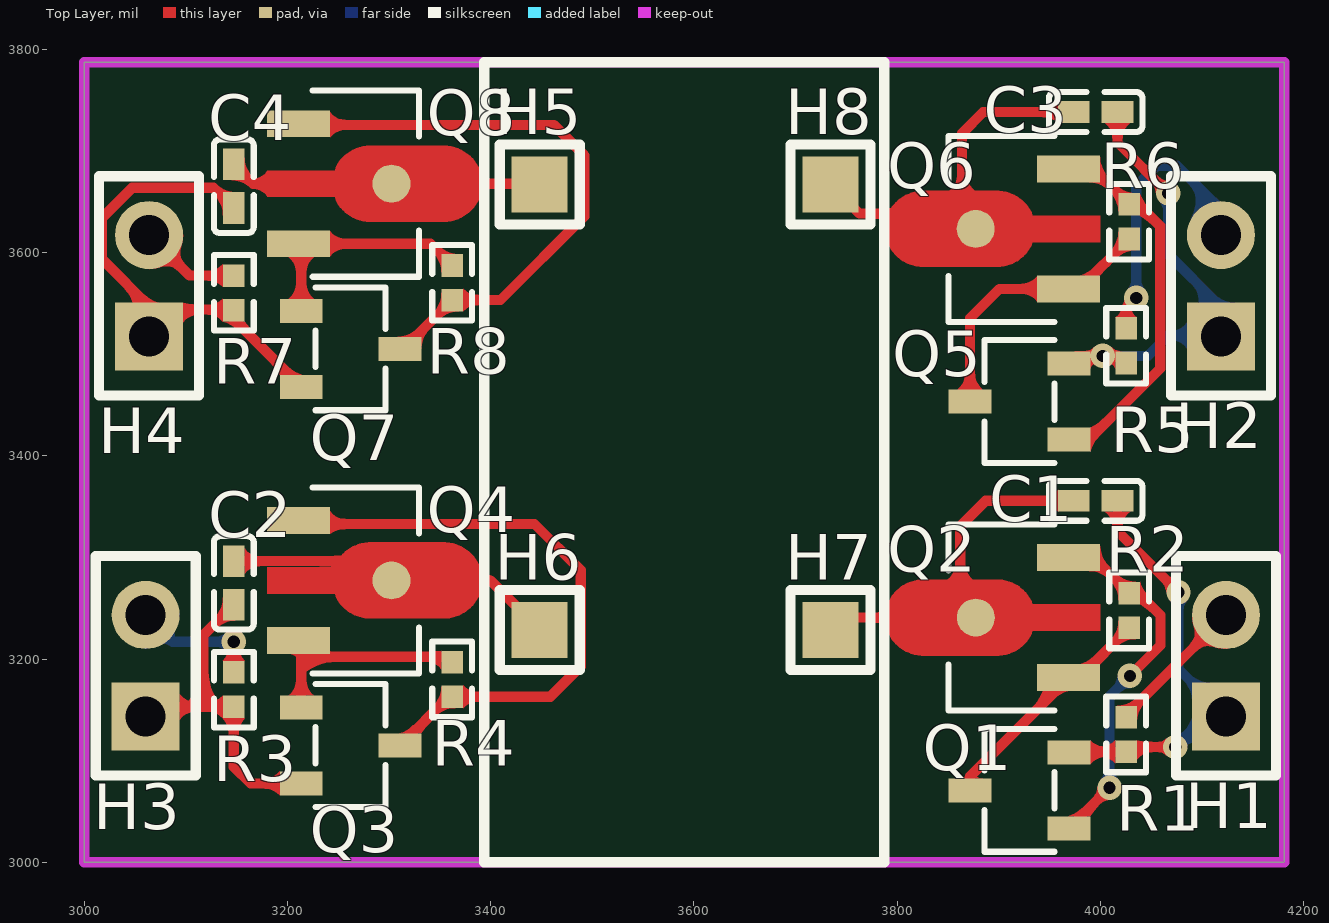
[diagram p0: Top Layer view]
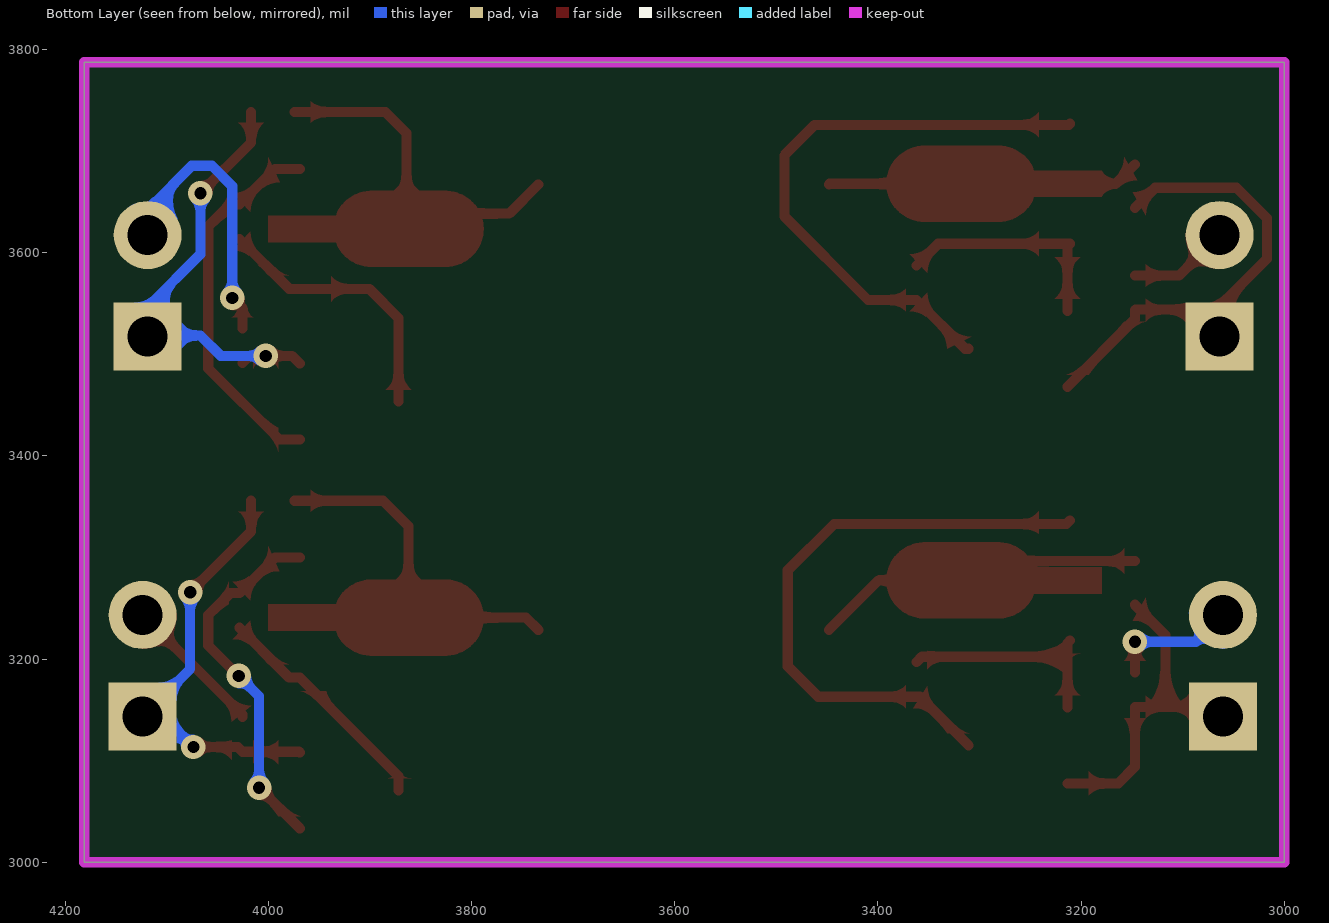
[diagram p1: Bottom Layer view, seen from below]
# Altium PCB MISC51349.pcbdoc
Units mil, origin at the board's own origin, x right, y up, seen from the top; angles counter-clockwise.
Board outline 1181.1 x 787.4 mil, 2 copper layers (Top Layer, Bottom Layer), stack 62.206 mil thick; 28 components, 20 nets, 60 pads, 8 vias.

## Layer stack, top to bottom
Top Solder Mask Layer: solder mask 0.394, Dk 3.3
Top Layer: signal copper 1.379
Dielectric1: surface 59.449, FR4, Dk 4.5
Bottom Layer: signal copper 1.378
Bottom Solder Mask Layer: solder mask 0.394, Dk 3.3

## Board outline
4181.1,3787.4 3000,3787.4 3000,3000 4181.1,3000

## Design rules (kind name [scope] priority, off if disabled: settings)
BoardOutlineClearance copperThickness2oz_1 [All] p2 off: genericclearance=7.99 ignorepadtopadclearanceinfootprint=FALSE except(0: Arc-SplitContinuation Track-SplitContinuation SMDPad-SplitContinuation THPad-SplitContinuation Via-SplitContinuation Fill-SplitContinuation Region-SplitContinuation Poly-SplitContinuation Text-SplitContinuation Hole-SplitContinuation; 5.98: Arc-CutoutEdge Track-CutoutEdge SMDPad-CutoutEdge THPad-CutoutEdge Via-CutoutEdge Text-CutoutEdge; 6.9: Hole-OutlineEdge Hole-CutoutEdge; 10: Poly-OutlineEdge Poly-CutoutEdge; 11.81: Arc-OutlineEdge Track-OutlineEdge SMDPad-OutlineEdge THPad-OutlineEdge Via-OutlineEdge Fill-OutlineEdge Region-OutlineEdge Text-OutlineEdge Fill-CutoutEdge Region-CutoutEdge)
BoardOutlineClearance Plane_innerPlane_1 [All] p4 off: genericclearance=4.02 ignorepadtopadclearanceinfootprint=FALSE except(0: Arc-SplitContinuation Track-SplitContinuation SMDPad-SplitContinuation THPad-SplitContinuation Via-SplitContinuation Fill-SplitContinuation Region-SplitContinuation Poly-SplitContinuation Text-SplitContinuation Hole-SplitContinuation; 5.98: Arc-CutoutEdge Track-CutoutEdge SMDPad-CutoutEdge THPad-CutoutEdge Via-CutoutEdge Text-CutoutEdge; 6.9: Hole-OutlineEdge Hole-CutoutEdge; 10: Poly-OutlineEdge Poly-CutoutEdge; 11.81: Arc-OutlineEdge Track-OutlineEdge SMDPad-OutlineEdge THPad-OutlineEdge Via-OutlineEdge Fill-OutlineEdge Region-OutlineEdge Text-OutlineEdge Fill-CutoutEdge Region-CutoutEdge)
BoardOutlineClearance Copper_copperRegion_1 [All] p6 off: genericclearance=4.02 ignorepadtopadclearanceinfootprint=FALSE except(0: Arc-SplitContinuation Track-SplitContinuation SMDPad-SplitContinuation THPad-SplitContinuation Via-SplitContinuation Fill-SplitContinuation Region-SplitContinuation Poly-SplitContinuation Text-SplitContinuation Hole-SplitContinuation; 5.98: Arc-CutoutEdge Track-CutoutEdge SMDPad-CutoutEdge THPad-CutoutEdge Via-CutoutEdge Text-CutoutEdge; 6.9: Hole-OutlineEdge Hole-CutoutEdge; 10: Poly-OutlineEdge Poly-CutoutEdge; 11.81: Arc-OutlineEdge Track-OutlineEdge SMDPad-OutlineEdge THPad-OutlineEdge Via-OutlineEdge Fill-OutlineEdge Region-OutlineEdge Text-OutlineEdge Fill-CutoutEdge Region-CutoutEdge)
BoardOutlineClearance copperThickness1oz_1 [All] p8: genericclearance=4.02 ignorepadtopadclearanceinfootprint=FALSE except(0: Arc-SplitContinuation Track-SplitContinuation SMDPad-SplitContinuation THPad-SplitContinuation Via-SplitContinuation Fill-SplitContinuation Region-SplitContinuation Poly-SplitContinuation Text-SplitContinuation Hole-SplitContinuation; 5.98: Arc-CutoutEdge Track-CutoutEdge SMDPad-CutoutEdge THPad-CutoutEdge Via-CutoutEdge Text-CutoutEdge; 6.9: Hole-OutlineEdge Hole-CutoutEdge; 10: Poly-OutlineEdge Poly-CutoutEdge; 11.81: Arc-OutlineEdge Track-OutlineEdge SMDPad-OutlineEdge THPad-OutlineEdge Via-OutlineEdge Fill-OutlineEdge Region-OutlineEdge Text-OutlineEdge Fill-CutoutEdge Region-CutoutEdge)
Clearance copperThickness2oz [All] p1 off: gap=7.99 ignorepadtopadclearanceinfootprint=FALSE except(5.98: SMDPad-Track SMDPad-SMDPad THPad-Track SMDPad-THPad THPad-THPad Track-Via SMDPad-Via THPad-Via Via-Via Fill-SMDPad Region-SMDPad Fill-THPad Region-THPad Fill-Via Region-Via Fill-Fill Fill-Region Region-Region Arc-Track Arc-SMDPad Arc-THPad Arc-Via Fill-Arc Region-Arc Arc-Arc Text-Track SMDPad-Text Text-THPad Text-Via Fill-Text Region-Text Arc-Text Text-Text; 6.9: Hole-Track Hole-SMDPad Hole-THPad Hole-Via Fill-Hole Region-Hole Hole-Arc Hole-Text; 10: Poly-Track Poly-SMDPad Poly-THPad Poly-Via Poly-Fill Poly-Region Poly-Poly Poly-Arc Poly-Text Poly-Hole; 11.81: Fill-Track Region-Track)
Clearance Plane_innerPlane [All] p3 off: gap=4.02 ignorepadtopadclearanceinfootprint=FALSE except(5.98: SMDPad-Track SMDPad-SMDPad THPad-Track SMDPad-THPad THPad-THPad Track-Via SMDPad-Via THPad-Via Via-Via Fill-SMDPad Region-SMDPad Fill-THPad Region-THPad Fill-Via Region-Via Fill-Fill Fill-Region Region-Region Arc-Track Arc-SMDPad Arc-THPad Arc-Via Fill-Arc Region-Arc Arc-Arc Text-Track SMDPad-Text Text-THPad Text-Via Fill-Text Region-Text Arc-Text Text-Text; 6.9: Hole-Track Hole-SMDPad Hole-THPad Hole-Via Fill-Hole Region-Hole Hole-Arc Hole-Text; 10: Poly-Track Poly-SMDPad Poly-THPad Poly-Via Poly-Fill Poly-Region Poly-Poly Poly-Arc Poly-Text Poly-Hole; 11.81: Fill-Track Region-Track)
Clearance Copper_copperRegion [All] p5 off: gap=4.02 ignorepadtopadclearanceinfootprint=FALSE except(5.98: SMDPad-Track SMDPad-SMDPad THPad-Track SMDPad-THPad THPad-THPad Track-Via SMDPad-Via THPad-Via Via-Via Fill-SMDPad Region-SMDPad Fill-THPad Region-THPad Fill-Via Region-Via Fill-Fill Fill-Region Region-Region Arc-Track Arc-SMDPad Arc-THPad Arc-Via Fill-Arc Region-Arc Arc-Arc Text-Track SMDPad-Text Text-THPad Text-Via Fill-Text Region-Text Arc-Text Text-Text; 6.9: Hole-Track Hole-SMDPad Hole-THPad Hole-Via Fill-Hole Region-Hole Hole-Arc Hole-Text; 10: Poly-Track Poly-SMDPad Poly-THPad Poly-Via Poly-Fill Poly-Region Poly-Poly Poly-Arc Poly-Text Poly-Hole; 11.81: Fill-Track Region-Track)
Clearance copperThickness1oz [All] p7: gap=4.02 ignorepadtopadclearanceinfootprint=FALSE except(5.98: SMDPad-Track SMDPad-SMDPad THPad-Track SMDPad-THPad THPad-THPad Track-Via SMDPad-Via THPad-Via Via-Via Fill-SMDPad Region-SMDPad Fill-THPad Region-THPad Fill-Via Region-Via Fill-Fill Fill-Region Region-Region Arc-Track Arc-SMDPad Arc-THPad Arc-Via Fill-Arc Region-Arc Arc-Arc Text-Track SMDPad-Text Text-THPad Text-Via Fill-Text Region-Text Arc-Text Text-Text; 6.9: Hole-Track Hole-SMDPad Hole-THPad Hole-Via Fill-Hole Region-Hole Hole-Arc Hole-Text; 10: Poly-Track Poly-SMDPad Poly-THPad Poly-Via Poly-Fill Poly-Region Poly-Poly Poly-Arc Poly-Text Poly-Hole; 11.81: Fill-Track Region-Track)
DiffPairsRouting differentialPair [All] p1: maxlimit=6 minlimit=6 mostfreqgap=6 toplayer_minwidth=5 toplayer_prefwidth=10 toplayer_maxwidth=100 toplayer_mingap=6 toplayer_prefgap=6 toplayer_maxgap=6 bottomlayer_minwidth=5 bottomlayer_prefwidth=10 bottomlayer_maxwidth=100 bottomlayer_mingap=6 bottomlayer_prefgap=6 bottomlayer_maxgap=6 maxuncoupledlength=10
HoleToHoleClearance otherClearance [All] p1: gap=11.81 allowstackedmicrovias=TRUE
Length netLength [All] p1: minlimit=0 maxlimit=0
PasteMaskExpansion pasteMaskExpansion [All] p1: expansion=0
PlaneConnect innerPlane [All] p1: planeconnectstyle=Relief reliefexpansion=20 reliefentries=4 reliefconductorwidth=10 reliefairgap=10
PolygonConnect copperRegion [All] p1: connectstyle=Relief reliefconductorwidth=10 reliefentries=4 polygonreliefangle="90 Angle" airgapwidth=10 via.connectstyle=Relief via.reliefconductorwidth=10 via.reliefentries=4 via.polygonreliefangle="90 Angle" via.airgapwidth=10
RoutingVias viaSize [All] p1: holewidth=12.01 width=24.02 viastyle="Through Hole" minholewidth=11.81 minwidth=19.68 maxholewidth=248.03 maxwidth=393.7
SolderMaskExpansion solderMaskExpansion [IsVia] p1: expansion=-1000 istentingtop=TRUE
SolderMaskExpansion solderMaskExpansion [All] p2: expansion=2 istentingtop=FALSE
Width copperThickness2oz_2 [All] p1 off: maxlimit=100 minlimit=8 preferedwidth=10
Width copperThickness1oz_2 [All] p2: maxlimit=100 minlimit=5 preferedwidth=10

## Components (designator, comment, footprint, x,y, rotation, side; value= is the part's Value field where it differs from the comment)
C1 "1nF" C0402 3995.47,3355.85 r0 top
C2 "1nF" C0402 3147.11,3275 r270 top
C3 "1nF" C0402 3995.43,3738.48 r0 top
C4 "1nF" C0402 3147.11,3665.43 r270 top
H1 "" HDR-TH_2P-P2.54-V-F 4123.7,3193.48 r90 top
H2 "" HDR-TH_2P-P2.54-V-F 4118.7,3567.4 r90 top
H3 "" HDR-TH_2P-P2.54-V-F 3060.43,3193.48 r90 top
H4 "" HDR-TH_2P-P2.54-V-F 3063.7,3567.4 r90 top
H5 "" HDR-TH_1P-V-M_XKB_X4611WV-01I-C28D40 3448.23,3667.09 r0 top
H6 "" HDR-TH_1P-V-M_XKB_X4611WV-01I-C28D40 3448.23,3228.78 r0 top
H7 "" HDR-TH_1P-V-M_XKB_X4611WV-01I-C28D40 3734.37,3228.78 r0 top
H8 "" HDR-TH_1P-V-M_XKB_X4611WV-01I-C28D40 3734.37,3667.09 r0 top
Q1 "BC856B" SOT-23-3_L2.9-W1.6-P1.90-LS2.8-BR 3920.47,3070.85 r0 top
Q2 "2N2222AU" SOT-89-3_L4.5-W2.4-P1.50-LS4.0-BR 3915.47,3240.85 r0 top
Q3 "BC856B" SOT-23-3_L2.9-W1.6-P1.90-LS2.8-BR 3262.11,3115 r180 top
Q4 "2N2222AU" SOT-89-3_L4.5-W2.4-P1.50-LS4.0-BR 3264.33,3277.5 r180 top
Q5 "BC856B" SOT-23-3_L2.9-W1.6-P1.90-LS2.8-BR 3920.43,3453.48 r0 top
Q6 "2N2222AU" SOT-89-3_L4.5-W2.4-P1.50-LS4.0-BR 3915.43,3623.48 r0 top
Q7 "BC856B" SOT-23-3_L2.9-W1.6-P1.90-LS2.8-BR 3262.11,3505.43 r180 top
Q8 "2N2222AU" SOT-89-3_L4.5-W2.4-P1.50-LS4.0-BR 3264.33,3667.93 r180 top
R1 "3.9K" R0402 4025.47,3125.85 r270 top
R2 "200k" R0402 4028.43,3247.89 r90 top
R3 "3.9K" R0402 3147.11,3170 r270 top
R4 "200k" R0402 3362.11,3180 r90 top
R5 "3.9K" R0402 4025.43,3508.48 r270 top
R6 "200k" R0402 4028.39,3630.52 r90 top
R7 "3.9K" R0402 3147.11,3560.43 r270 top
R8 "200k" R0402 3362.11,3570.43 r90 top

## Footprints (in the part's own frame and the unit in brackets; to place one, negate y for a bottom-side part, rotate by r counter-clockwise, add the part's x,y. Pads: shape width x height; smd on the part's side, far side on the other; paste and mask are expansions set on the pad)
C0402 [mm]
  rect 0.79x0.54 smd paste-100 mask+0.051: 1(-0.545,0) 2(0.545,0)
  silkscreen extent -1.17,-0.5 1.17,0.5
HDR-TH_1P-V-M_XKB_X4611WV-01I-C28D40 [mm]
  rect 1.4x1.4 smd: 1(0,0)
  silkscreen extent -1,-1 1,1
HDR-TH_2P-P2.54-V-F [mm]
  rect 1.7x1.7 hole 1: 1(-1.27,0)
  round 1.7 hole 1: 2(1.27,0)
  silkscreen extent -2.74,-1.25 2.74,1.25
R0402 [mm]
  rect 0.566x0.54 smd paste-100 mask+0.051: 1(-0.433,0) 2(0.433,0)
  silkscreen extent -0.94,-0.5 0.94,0.5
SOT-23-3_L2.9-W1.6-P1.90-LS2.8-BR [mm]
  rect 1.07x0.6 smd: 1(1.235,-0.95) 2(1.235,0.95) 3(-1.235,0)
  silkscreen extent -0.88,-1.54 0.88,1.54
SOT-89-3_L4.5-W2.4-P1.50-LS4.0-BR [mm]
  rect 1.575x0.672 smd: 1(1.356,-1.5) 3(1.356,1.5)
  round 0.95 smd: 2(-0.966,0)
  Top Layer region: -2.283,0.95 -0.429,0.95 -0.384,0.949 -0.34,0.946 -0.296,0.941 -0.252,0.933 -0.208,0.924 -0.165,0.913 -0.123,0.899 -0.081,0.884 -0.04,0.867 0,0.847 0.04,0.826 0.078,0.804 0.115,0.779 0.151,0.753 0.185,0.725 0.219,0.695 0.251,0.664 0.281,0.631 0.31,0.597 0.337,0.562 0.362,0.525 0.386,0.488 0.408,0.449 0.428,0.409 0.447,0.33 2.144,0.33 2.144,-0.33 0.447,-0.33 0.428,-0.409 0.408,-0.449 0.386,-0.488 0.362,-0.525 0.337,-0.562 0.31,-0.597 0.281,-0.631 0.251,-0.664 0.219,-0.695 0.185,-0.725 0.151,-0.753 0.115,-0.779 0.078,-0.804 0.04,-0.826 0,-0.847 -0.04,-0.867 -0.081,-0.884 -0.123,-0.899 -0.165,-0.913 -0.208,-0.924 -0.252,-0.933 -0.296,-0.941 -0.34,-0.946 -0.384,-0.949 -0.429,-0.95 -2.283,-0.95 -2.328,-0.949 -2.372,-0.946 -2.416,-0.941 -2.46,-0.933 -2.504,-0.924 -2.547,-0.913 -2.589,-0.899 -2.631,-0.884 -2.672,-0.867 -2.712,-0.847 -2.752,-0.826 -2.79,-0.804 -2.827,-0.779 -2.863,-0.753 -2.898,-0.725 -2.931,-0.695 -2.963,-0.664 -2.993,-0.631 -3.022,-0.597 -3.049,-0.562 -3.075,-0.525 -3.098,-0.488 -3.12,-0.449 -3.14,-0.409 -3.159,-0.369 -3.175,-0.327 -3.189,-0.285 -3.202,-0.242 -3.212,-0.199 -3.22,-0.155 -3.227,-0.111 -3.231,-0.067 -3.233,-0.022 -3.233,0.022 -3.231,0.067 -3.227,0.111 -3.22,0.155 -3.212,0.199 -3.202,0.242 -3.189,0.285 -3.175,0.327 -3.159,0.369 -3.14,0.409 -3.12,0.449 -3.098,0.488 -3.075,0.525 -3.049,0.562 -3.022,0.597 -2.993,0.631 -2.963,0.664 -2.931,0.695 -2.898,0.725 -2.863,0.753 -2.827,0.779 -2.79,0.804 -2.752,0.826 -2.712,0.847 -2.672,0.867 -2.631,0.884 -2.589,0.899 -2.547,0.913 -2.504,0.924 -2.46,0.933 -2.416,0.941 -2.372,0.946 -2.328,0.949
  silkscreen extent -1.65,-2.33 1,2.33

## Via types
v1: diameter 24.02, hole 12, Top Layer to Bottom Layer, 8 vias

## Nets (pads, with @x,y where several pads share a name; then routed paths per layer and width w, separated by ;. In a path a pad name is that pad's centre, name@x,y a point inside that pad or via, vN(x,y) a via of type N, cw(c..) or ccw(c..) an arc to the next point about the centre after c; other vN are vias at no path point)
$1N629: Q1.3 Q2.1 R2.1 | length 231
  Top Layer w10: Q1.3 3871.84,3084.77 Q2.1 3979.38,3181.8 R2.1
$1N634: Q1.1 Q2.3 R2.2 | length 360.9
  Top Layer w10: Q2.3 3993.45,3299.91 R2.2 4037.61,3264.93 4059.09,3243.45 4059.09,3213.45 v1(4029.09,3183.45) ; Q1.1 v1(4009.09,3073.45)
  Bottom Layer w10: v1(4009.09,3073.45) 4009.09,3163.45 v1(4029.09,3183.45)
$1N1172: Q3.3 Q4.1 R4.1 | length 602.8
  Top Layer w10: Q4.1 3214.52,3332.96 3443.14,3332.96 3488.69,3287.41 3488.69,3192.96 3458.69,3162.96 3358.69,3162.96 Q3.3
$1N1177: Q3.1 Q4.3 R4.2 | length 217.9
  Top Layer w10: Q4.3 3213.48,3215.89 3213.48,3202.4 ; Q3.1 3213.48,3202.4 ; R4.2 3356.75,3202.4 3213.48,3202.4
$1N1509: Q5.3 Q6.1 R6.1 | length 270.9
  Top Layer w10: Q5.3 3871.8,3535.5 3900.73,3564.43 Q6.1 3979.34,3564.43 R6.1
$1N1514: Q5.1 Q6.3 R6.2 | length 372.6
  Top Layer w10: Q6.3 3993.41,3682.54 R6.2 4037.57,3647.56 4059.05,3626.08 4059.05,3486.08 3989.05,3416.08 Q5.1
$1N1525: Q7.3 Q8.1 R8.1 | length 589.5
  Top Layer w10: Q8.1 3212.11,3725.81 3462.11,3725.81 3492.11,3695.81 3492.11,3635.81 3409.69,3553.39 R8.1 3314.15,3505.43 Q7.3
$1N1530: Q7.1 Q8.3 R8.2 | length 227.1
  Top Layer w10: Q7.1 3213.48,3606.32 Q8.3 3340.7,3608.87 R8.2
V1: C1.2 H1.1 Q1.2 R1.2 | length 425.8
  Top Layer w10: Q1.2 3969.65,3108.81 R1.2 4030.14,3113.48 v1(4073.7,3113.48) ; C1.2 4016.93,3325.85 v1(4076.93,3265.85)
  Bottom Layer w10: v1(4073.7,3113.48) 4103.7,3143.48 H1.1 4076.93,3190.26 v1(4076.93,3265.85)
V2: C3.2 H2.1 Q5.2 R5.2 | length 448.7
  Top Layer w10: Q5.2 3976.65,3498.48 v1(4002.47,3498.48) 4018.39,3498.48 R5.2 ; C3.2 4016.89,3708.48 v1(4066.89,3658.48)
  Bottom Layer w10: v1(4002.47,3498.48) 4046.89,3498.48 4066.89,3518.48 H2.1@4116.89,3518.48 ; v1(4066.89,3658.48) 4066.89,3598.48 4116.89,3548.48 H2.1@4116.89,3518.48 ; H2.1 H2.1@4116.89,3518.48
V3: C2.2 H3.1 Q3.2 R3.2 | length 335.7
  Top Layer w10: H3.1 3069.9,3152.96 3117.11,3152.96 ; C2.2 3117.11,3223.54 3117.11,3152.96 ; Q3.2 3163.5,3077.6 3147.11,3094 R3.2 3117.11,3152.96
V4: C4.2 H4.1 Q7.2 R7.2 | length 472.5
  Top Layer w10: H4.1 3067.11,3520.81 H4.1@3067.11,3543.97 ; C4.2 3127.11,3663.97 3047.11,3663.97 3017.11,3633.97 3017.11,3593.97 H4.1@3067.11,3543.97 ; Q7.2 3147.11,3534.4 R7.2 3146.53,3543.97 H4.1@3067.11,3543.97
VIN1: H1.2 R1.1 | length 141.3
  Top Layer w10: R1.1 4025.47,3145.25 H1.2
VIN2: H2.2 R5.1 | length 278.5
  Top Layer w10: R5.1 4025.43,3545.52 v1(4035.43,3555.52)
  Bottom Layer w10: v1(4035.43,3555.52) 4035.43,3665.52 4055.43,3685.52 4075.43,3685.52 4115.43,3645.52 4115.43,3620.68 H2.2
VIN3: H3.2 R3.1 | length 127.6
  Top Layer w10: R3.1 v1(3147.11,3217.04)
  Bottom Layer w10: H3.2 3086.87,3217.04 v1(3147.11,3217.04)
VIN4: H4.2 R7.1 | length 99.9
  Top Layer w10: H4.2 3103.63,3577.47 R7.1
VOUT1: C1.1 H7.1 Q2.2 | length 345
  Top Layer w10: H7.1 3746.43,3240.84 3862.07,3240.84 3862.07,3330.77 3887.15,3355.85 C1.1
VOUT2: C3.1 H8.1 Q6.2 | length 355.1
  Top Layer w10: H8.1 3762.97,3638.48 3863.97,3638.48 ; Q6.2@3862.03,3623.47 3863.97,3625.41 3863.97,3638.48 ; C3.1 3884.78,3738.48 3863.97,3717.67 3863.97,3638.48
VOUT3: C2.1 H6.1 Q4.2 | length 329.2
  Top Layer w10: C2.1 3298.78,3296.46 3317.73,3277.51 3399.49,3277.51 H6.1
VOUT4: C4.1 H5.1 Q8.2 | length 309.3
  Top Layer w10: C4.1 3166.05,3667.94 3317.73,3667.94 3447.37,3667.94 H5.1

## Keep-outs
Board Outline Layer:
  the board outline again, w10

## Other copper
Top Layer:
  region net V1: 4021.93,3330.22 4011.93,3330.22 4011.61,3333.68 4010.65,3337.02 4009.1,3340.12 4007,3342.89 4004.43,3345.22 4029.43,3345.22 4026.86,3342.89 4024.76,3340.12 4023.2,3337.02 4022.25,3333.68 4021.93,3330.22
  region net VOUT1: 3943.46,3350.85 3943.46,3360.85 3947.53,3361.22 3951.47,3362.3 3955.15,3364.08 3958.46,3366.48 3958.46,3345.22 3955.15,3347.62 3951.47,3349.4 3947.53,3350.48 3943.46,3350.85
  region net V3: 3133.32,3232.68 3131.17,3244.68 3133.45,3248.28 3135.11,3252.2 3136.13,3256.34 3136.48,3260.59 3149.23,3237.99 3144.98,3237.64 3140.84,3236.63 3136.92,3234.96 3133.32,3232.68
  region net VOUT3: 3172.74,3301.46 3172.74,3291.46 3169.28,3291.14 3165.94,3290.18 3162.83,3288.63 3160.07,3286.53 3157.74,3283.96 3157.74,3308.96 3160.07,3306.39 3162.83,3304.29 3165.94,3302.74 3169.28,3301.78 3172.74,3301.46
  region net V2: 4021.89,3712.85 4011.89,3712.85 4011.56,3716.31 4010.61,3719.65 4009.06,3722.76 4006.96,3725.52 4004.39,3727.85 4029.39,3727.85 4026.81,3725.52 4024.71,3722.76 4023.16,3719.65 4022.21,3716.31 4021.89,3712.85
  region net VOUT2: 3943.41,3733.48 3943.41,3743.48 3947.48,3743.85 3951.42,3744.94 3955.11,3746.71 3958.41,3749.11 3958.41,3727.85 3955.11,3730.26 3951.42,3732.03 3947.48,3733.12 3943.41,3733.48
  region net V4: 3131.17,3652.83 3133.32,3664.83 3136.92,3662.55 3140.84,3660.88 3144.98,3659.87 3149.23,3659.52 3136.48,3636.92 3136.13,3641.17 3135.11,3645.31 3133.45,3649.23 3131.17,3652.83
  region net VOUT4: 3163.04,3678.03 3160.89,3666.03 3157.29,3668.31 3153.37,3669.98 3149.23,3670.99 3144.98,3671.34 3157.74,3693.94 3158.08,3689.69 3159.1,3685.55 3160.76,3681.63 3163.04,3678.03
  region net $1N634: 3981.73,3053.15 3999.67,3056.96 3994.61,3051.35 3990.16,3045.26 3968.4,3045.26 3972.08,3046.59 3975.56,3048.37 3978.79,3050.57 3981.73,3053.15
  region net V1: 4005.16,3113.81 4005.16,3103.81 4001.71,3103.49 3998.39,3102.56 3995.28,3101.03 3992.51,3098.97 3990.16,3096.44 3990.16,3120.06 3992.68,3117.89 3995.52,3116.14 3998.59,3114.86 4001.83,3114.07 4005.16,3113.81
  region net $1N629: 3866.84,3084.77 3876.84,3084.77 3879.2,3083.61 3881.73,3082.9 3884.34,3082.66 3859.34,3082.66 3861.96,3082.9 3864.49,3083.61 3866.84,3084.77
  region net $1N634: 4005.18,3295.25 4004.91,3281.38 4001.31,3283.65 3997.38,3285.32 3993.25,3286.34 3989,3286.68 3999.88,3311.16 4000.22,3306.91 4001.24,3302.78 4002.9,3298.85 4005.18,3295.25
  region net $1N629: 3954.82,3160.68 3935.25,3155.25 3937.84,3158.18 3940.04,3161.41 3941.81,3164.9 3943.14,3168.57 3968.14,3168.57 3964.47,3167.24 3960.99,3165.46 3957.75,3163.27 3954.82,3160.68
  region net $1N629: 3993.43,3202.92 4010.38,3205.73 4005.1,3200.41 3999.88,3195.03 3980.11,3195.03 3983.78,3196.36 3987.26,3198.14 3990.5,3200.33 3993.43,3202.92
  region net $1N1177: 3208.48,3179.21 3218.48,3179.21 3218.8,3175.75 3219.76,3172.41 3221.31,3169.31 3223.41,3166.54 3225.98,3164.21 3200.98,3164.21 3203.55,3166.54 3205.65,3169.31 3207.21,3172.41 3208.16,3175.75 3208.48,3179.21
  region net V3: 3177.42,3072.6 3177.42,3082.6 3180.8,3082.89 3184.08,3083.75 3187.17,3085.15 3189.98,3087.06 3192.42,3089.41 3192.42,3065.79 3189.98,3068.14 3187.17,3070.05 3184.08,3071.45 3180.8,3072.31
  region net $1N1172: 3323.36,3134.7 3341.31,3138.51 3336.25,3132.9 3331.79,3126.81 3310.04,3126.81 3313.72,3128.14 3317.2,3129.92 3320.43,3132.12 3323.36,3134.7
  region net $1N1177: 3218.48,3202.4 3208.48,3202.4 3206.23,3203.93 3203.68,3204.89 3200.98,3205.21 3225.98,3205.21 3223.28,3204.89 3220.73,3203.93 3218.48,3202.4
  region net $1N1172: 3256.93,3337.96 3256.93,3327.96 3252.97,3327.66 3249.08,3326.77 3245.38,3325.32 3241.93,3323.32 3241.93,3345.46 3244.27,3342.89 3247.03,3340.79 3250.14,3339.24 3253.48,3338.28 3256.93,3337.96
  region net $1N1514: 4002.56,3436.66 3997.82,3417.78 3995.23,3414.82 3993.06,3411.54 3991.34,3408.01 3990.11,3404.27 3990.11,3427.89 3994.59,3430.33 3998.75,3433.27 4002.56,3436.66
  region net V2: 4002.47,3503.48 4002.47,3493.48 3999.45,3493.15 3996.58,3492.18 3993.99,3490.6 3991.8,3488.51 3990.11,3485.98 3990.11,3502.69 3996.3,3502.89 4002.47,3503.48
  region net $1N1509: 3866.8,3480.29 3876.8,3480.29 3877.12,3476.84 3878.08,3473.5 3879.63,3470.39 3881.73,3467.63 3884.3,3465.29 3859.3,3465.29 3861.87,3467.63 3863.97,3470.39 3865.53,3473.5 3866.48,3476.84 3866.8,3480.29
  region net $1N1514: 4005.14,3677.88 4004.87,3664.01 4001.26,3666.29 3997.34,3667.95 3993.2,3668.97 3988.96,3669.31 3999.83,3693.79 4000.17,3689.55 4001.19,3685.41 4002.86,3681.49 4005.14,3677.88
  region net $1N1509: 3922.82,3559.43 3922.82,3569.43 3926.28,3569.75 3929.62,3570.71 3932.73,3572.26 3935.49,3574.36 3937.82,3576.93 3937.82,3551.93 3935.49,3554.51 3932.73,3556.61 3929.62,3558.16 3926.28,3559.11 3922.82,3559.43
  region net $1N1509: 3993.38,3585.55 4010.34,3588.37 4005.06,3583.04 3999.83,3577.66 3980.06,3577.66 3983.74,3578.99 3987.22,3580.77 3990.45,3582.97 3993.38,3585.55
  region net $1N1530: 3208.48,3569.64 3218.48,3569.64 3218.8,3566.18 3219.76,3562.84 3221.31,3559.74 3223.41,3556.97 3225.98,3554.64 3200.98,3554.64 3203.55,3556.97 3205.65,3559.74 3207.21,3562.84 3208.16,3566.18 3208.48,3569.64
  region net V4: 3182.9,3491.54 3200.85,3487.73 3203.78,3485.15 3207.01,3482.95 3210.49,3481.17 3214.17,3479.84 3192.42,3479.84 3187.96,3485.93 3182.9,3491.54
  region net $1N1525: 3324.19,3522.54 3337.1,3521.31 3334.82,3517.71 3333.15,3513.79 3332.14,3509.65 3331.79,3505.4 3308.28,3517.24 3312.53,3517.58 3316.66,3518.6 3320.59,3520.27 3324.19,3522.54
  region net $1N1530: 3218.48,3580.64 3208.48,3580.64 3208.16,3584.1 3207.21,3587.44 3205.65,3590.55 3203.55,3593.31 3200.98,3595.64 3225.98,3595.64 3223.41,3593.31 3221.31,3590.55 3219.76,3587.44 3218.8,3584.1 3218.48,3580.64
  region net $1N1530: 3256.93,3613.87 3256.93,3603.87 3253.48,3603.55 3250.14,3602.6 3247.03,3601.04 3244.27,3598.95 3241.93,3596.37 3241.93,3621.37 3244.27,3618.8 3247.03,3616.7 3250.14,3615.15 3253.48,3614.19 3256.93,3613.87
  region net $1N1525: 3256.93,3730.81 3256.93,3720.81 3253.53,3720.51 3250.23,3719.62 3247.13,3718.16 3244.34,3716.19 3241.93,3713.75 3241.93,3738.31 3244.27,3735.73 3247.03,3733.64 3250.14,3732.08 3253.48,3731.13 3256.93,3730.81
  region net V1: 3999.84,3103.81 3999.84,3113.81 4003.15,3114.07 4006.38,3114.83 4009.45,3116.09 4012.3,3117.81 4014.84,3119.95 4014.84,3097.68 4012.3,3099.81 4009.45,3101.53 4006.38,3102.79 4003.15,3103.55 3999.84,3103.81
  region net V1: 4051.1,3118.48 4051.1,3108.48 4047.64,3108.16 4044.3,3107.21 4041.2,3105.66 4038.43,3103.56 4036.1,3100.98 4036.1,3119.95 4043.56,3118.85 4051.1,3118.48
  region net VIN1: 4032.47,3159.33 4041.4,3154.11 4039.13,3150.51 4037.46,3146.59 4036.44,3142.45 4036.1,3138.2 4016.57,3154.03 4020.81,3154.37 4024.95,3155.39 4028.87,3157.05 4032.47,3159.33
  region net $1N634: 4012.5,3273.79 4019.06,3281.37 4022.66,3279.09 4026.59,3277.43 4030.72,3276.41 4034.97,3276.07 4017.8,3257.88 4017.46,3262.13 4016.44,3266.27 4014.77,3270.19 4012.5,3273.79
  region net $1N634: 4046.91,3262.7 4050.97,3244.5 4047.26,3247.92 4043.28,3251.03 4039.06,3253.8 4039.06,3276.07 4040.37,3272.38 4042.13,3268.88 4044.32,3265.64 4046.91,3262.7
  region net $1N629: 4019.06,3214.41 4012.5,3221.99 4014.77,3225.59 4016.44,3229.51 4017.46,3233.65 4017.8,3237.9 4034.97,3219.72 4030.72,3219.37 4026.59,3218.35 4022.66,3216.69 4019.06,3214.41
  region net V3: 3152.11,3126.82 3142.11,3126.82 3141.74,3130.9 3140.65,3134.84 3138.88,3138.52 3136.48,3141.82 3157.74,3141.82 3155.33,3138.52 3153.56,3134.84 3152.47,3130.9 3152.11,3126.82
  region net V3: 3121.48,3147.96 3121.48,3157.96 3124.79,3158.22 3128.02,3158.98 3131.09,3160.24 3133.93,3161.96 3136.48,3164.09 3136.48,3141.82 3133.93,3143.96 3131.09,3145.68 3128.02,3146.94 3124.79,3147.7 3121.48,3147.96
  region net VIN3: 3142.11,3213.18 3152.11,3213.18 3152.47,3209.1 3153.56,3205.16 3155.33,3201.48 3157.74,3198.18 3136.48,3198.18 3138.88,3201.48 3140.65,3205.16 3141.74,3209.1 3142.11,3213.18
  region net $1N1177: 3336.48,3197.4 3336.48,3207.4 3343.99,3207.59 3351.48,3208.18 3351.48,3189.9 3349.14,3192.47 3346.38,3194.57 3343.27,3196.12 3339.93,3197.08 3336.48,3197.4
  region net $1N1172: 3349.32,3146.52 3346.17,3157.51 3348.45,3161.12 3350.11,3165.04 3351.13,3169.18 3351.48,3173.42 3365.23,3151.82 3360.99,3151.48 3356.85,3150.46 3352.93,3148.8 3349.32,3146.52
  region net $1N1172: 3387.74,3167.96 3387.74,3157.96 3384.42,3157.7 3381.19,3156.94 3378.12,3155.68 3375.28,3153.96 3372.74,3151.82 3372.74,3174.09 3375.28,3171.96 3378.12,3170.24 3381.19,3168.98 3384.42,3168.22 3387.74,3167.96
  region net V2: 4002.47,3493.48 4002.47,3503.48 4008.61,3502.8 4014.8,3502.58 4014.8,3485.98 4013.12,3488.5 4010.93,3490.6 4008.34,3492.18 4005.48,3493.15 4002.47,3493.48
  region net VIN2: 4020.43,3545.52 4030.43,3545.52 4030.81,3542.79 4031.95,3540.27 4033.75,3538.17 4036.06,3536.66 4014.8,3536.66 4017.1,3538.17 4018.9,3540.27 4020.04,3542.79 4020.43,3545.52
  region net $1N1514: 4012.45,3656.43 4019.02,3664 4022.62,3661.73 4026.54,3660.06 4030.68,3659.04 4034.93,3658.7 4017.76,3640.52 4017.41,3644.76 4016.39,3648.9 4014.73,3652.82 4012.45,3656.43
  region net $1N1514: 4046.87,3645.34 4050.93,3627.13 4047.22,3630.55 4043.24,3633.66 4039.02,3636.43 4039.02,3658.7 4040.32,3655.01 4042.09,3651.52 4044.28,3648.27 4046.87,3645.34
  region net $1N1509: 4019.02,3597.04 4012.45,3604.62 4014.73,3608.22 4016.39,3612.15 4017.41,3616.28 4017.76,3620.53 4034.93,3602.35 4030.68,3602.01 4026.54,3600.99 4022.62,3599.32 4019.02,3597.04
  region net V4: 3121.48,3538.97 3121.48,3548.97 3125.54,3549.33 3129.47,3550.4 3133.16,3552.15 3136.48,3554.52 3136.48,3532.25 3134.02,3534.58 3131.21,3536.46 3128.12,3537.84 3124.85,3538.69 3121.48,3538.97
  region net V4: 3167.64,3520.94 3149.94,3524.5 3146.98,3527.09 3143.72,3529.27 3140.2,3531 3136.48,3532.25 3157.74,3532.25 3162.5,3526.44 3167.64,3520.94
  region net VIN4: 3121.48,3572.47 3121.48,3582.47 3124.79,3582.73 3128.02,3583.49 3131.09,3584.75 3133.93,3586.47 3136.48,3588.6 3136.48,3566.33 3133.93,3568.47 3131.09,3570.19 3128.02,3571.45 3124.79,3572.21 3121.48,3572.47
  region net $1N1530: 3346.17,3596.33 3352.74,3603.91 3356.34,3601.63 3360.26,3599.97 3364.4,3598.95 3368.65,3598.6 3351.48,3580.42 3351.13,3584.67 3350.11,3588.81 3348.45,3592.73 3346.17,3596.33
  region net $1N1525: 3387.74,3558.39 3387.74,3548.39 3384.42,3548.13 3381.19,3547.37 3378.12,3546.11 3375.28,3544.39 3372.74,3542.25 3372.74,3564.52 3375.28,3562.39 3378.12,3560.67 3381.19,3559.41 3384.42,3558.65 3387.74,3558.39
  region net $1N1525: 3352.74,3536.95 3346.17,3544.53 3348.45,3548.13 3350.11,3552.05 3351.13,3556.19 3351.48,3560.44 3368.65,3542.25 3364.4,3541.91 3360.26,3540.89 3356.34,3539.23 3352.74,3536.95
  region net VIN1: 4095.02,3207.73 4087.95,3214.8 4089.74,3216.75 4091.1,3218.59 4092.07,3220.33 4092.72,3222.01 4093.06,3223.65 4093.16,3225.26 4093.06,3226.88 4092.8,3228.53 4091.04,3235.88 4090.37,3240.34 4090.24,3242.85 4090.3,3245.58 4125.8,3210.08 4123.07,3210.02 4120.56,3210.15 4116.1,3210.83 4108.75,3212.58 4107.1,3212.84 4105.48,3212.95 4103.86,3212.85 4102.23,3212.5 4100.55,3211.86 4098.81,3210.88 4096.97,3209.52
  region net V3: 3108.89,3157.96 3108.89,3147.96 3105.43,3147.64 3102.09,3146.68 3098.99,3145.13 3096.22,3143.03 3093.89,3140.46 3093.89,3165.46 3096.22,3162.89 3098.99,3160.79 3102.09,3159.24 3105.43,3158.28 3108.89,3157.96
  region net V4: 3112.17,3548.97 3112.17,3538.97 3108.71,3538.65 3105.37,3537.69 3102.26,3536.14 3099.5,3534.04 3097.17,3531.47 3097.17,3550.87 3102.11,3549.82 3107.12,3549.18 3112.17,3548.97
  region net V4: 3039.82,3564.19 3059.39,3558.76 3062.32,3556.17 3065.55,3553.97 3069.03,3552.2 3072.71,3550.87 3047.71,3550.87 3046.38,3554.54 3044.6,3558.02 3042.4,3561.26 3039.82,3564.19
  region net VIN4: 3099.45,3588.72 3092.38,3581.65 3090.43,3583.44 3088.6,3584.8 3086.85,3585.78 3085.17,3586.42 3083.54,3586.76 3081.92,3586.86 3080.3,3586.76 3078.65,3586.5 3071.3,3584.74 3066.84,3584.07 3064.33,3583.94 3061.61,3584 3097.1,3619.5 3097.16,3616.77 3097.03,3614.26 3096.36,3609.8 3094.6,3602.45 3094.34,3600.8 3094.24,3599.18 3094.34,3597.57 3094.69,3595.93 3095.33,3594.25 3096.31,3592.51 3097.67,3590.67
  region net VOUT1: 3773.68,3235.84 3773.68,3245.84 3781.2,3246.12 3788.68,3246.96 3788.52,3245.84 3788.52,3235.84 3788.68,3234.74 3781.2,3235.56 3773.68,3235.84
  region net VOUT1: 3857.07,3293.25 3867.07,3293.25 3867.39,3289.79 3868.35,3286.46 3869.9,3283.35 3872,3280.58 3874.57,3278.25 3867.07,3278.25 3857.07,3278.25 3849.57,3278.25 3852.14,3280.58 3854.24,3283.35 3855.8,3286.46 3856.75,3289.79 3857.07,3293.25
  region net VOUT3: 3399.49,3282.51 3399.49,3272.51 3395.27,3272.23 3391.12,3271.39 3391.28,3272.51 3391.28,3282.51 3391.12,3283.61 3395.27,3282.79 3399.49,3282.51
  region net VOUT3: 3231.75,3291.46 3238.27,3301.46 3245.78,3301.68 3253.27,3302.36 3252.51,3301.46 3246.97,3291.46 3246.75,3290.49 3239.27,3291.22 3231.75,3291.46
  region net VOUT2: 3774.37,3633.48 3779.38,3643.48 3786.89,3643.66 3794.38,3644.17 3793.94,3643.48 3789.5,3633.48 3789.37,3633.02 3781.87,3633.37 3774.37,3633.48
  region net VOUT2: 3858.97,3675.89 3868.97,3675.89 3869.29,3672.43 3870.24,3669.09 3871.79,3665.98 3873.89,3663.22 3876.47,3660.89 3868.97,3660.89 3858.97,3660.89 3851.47,3660.89 3854.04,3663.22 3856.14,3665.98 3857.69,3669.09 3858.64,3672.43 3858.97,3675.89
  region net VOUT4: 3406.12,3672.94 3406.12,3662.94 3398.6,3662.66 3391.12,3661.82 3391.28,3662.94 3391.28,3672.94 3391.12,3674.04 3398.6,3673.22 3406.12,3672.94
  region net VOUT4: 3166.05,3662.94 3166.05,3672.94 3169.32,3673.27 3172.46,3674.23 3175.34,3675.79 3177.87,3677.89 3179.93,3680.44 3179.93,3672.94 3179.93,3662.94 3179.93,3655.44 3177.87,3658 3175.34,3660.1 3172.46,3661.66 3169.32,3662.62 3166.05,3662.94
  region net $1N634: 4001.07,3058.35 3994,3065.43 3994.74,3066.29 3995.36,3067.28 3996.29,3069.48 3996.84,3071.86 3997.11,3074.2 4009.85,3061.47 4007.5,3061.2 4005.13,3060.64 4002.92,3059.72 4001.94,3059.1
  region net V1: 4061.83,3273.87 4068.9,3280.95 4069.77,3280.2 4070.75,3279.58 4072.96,3278.66 4075.34,3278.1 4077.68,3277.83 4064.94,3265.1 4064.68,3267.44 4064.12,3269.82 4063.2,3272.02 4062.57,3273.01
  region net V1: 4057.35,3108.48 4057.35,3118.48 4058.49,3118.57 4059.62,3118.83 4061.84,3119.73 4063.91,3121.02 4065.76,3122.49 4065.76,3104.48 4063.91,3105.95 4061.84,3107.23 4059.62,3108.14 4058.49,3108.39
  region net V2: 4051.79,3666.51 4058.86,3673.58 4059.73,3672.84 4060.71,3672.22 4062.92,3671.29 4065.29,3670.73 4067.64,3670.47 4054.9,3657.73 4054.64,3660.08 4054.08,3662.45 4053.15,3664.66 4052.53,3665.64
  region net V2: 3986.12,3493.48 3986.12,3503.48 3987.25,3503.57 3988.39,3503.83 3990.6,3504.73 3992.68,3506.02 3994.52,3507.49 3994.52,3489.48 3992.68,3490.95 3990.6,3492.23 3988.39,3493.14 3987.25,3493.39
  region net V2: 4018.39,3503.48 4018.39,3493.48 4017.27,3493.39 4016.18,3493.14 4014.11,3492.23 4012.19,3490.95 4010.41,3489.48 4010.41,3507.49 4012.19,3506.02 4014.11,3504.73 4016.18,3503.83 4017.27,3503.57
  region net VIN2: 4028.96,3541.99 4021.89,3549.06 4022.56,3549.86 4023.01,3550.66 4023.27,3551.49 4023.4,3552.34 4023.44,3556.28 4036.18,3543.54 4032.24,3543.49 4031.39,3543.37 4030.57,3543.11 4029.76,3542.66
  region net VIN3: 3152.11,3200.69 3142.11,3200.69 3142.02,3201.83 3141.76,3202.96 3140.85,3205.18 3139.57,3207.25 3138.1,3209.1 3156.11,3209.1 3154.64,3207.25 3153.36,3205.18 3152.45,3202.96 3152.2,3201.83
  region net $1N1177: 3248.48,3197.4 3243.13,3197.11 3237.84,3196.25 3232.67,3194.83 3227.68,3192.87 3222.93,3190.38 3218.48,3187.4 3213.48,3202.4 3218.48,3215.89 3224.03,3212.89 3229.88,3210.51 3235.95,3208.79 3242.18,3207.75 3248.48,3207.4 3248.48,3197.4
  region net V3: 3112.11,3187.96 3111.82,3182.61 3110.96,3177.32 3109.54,3172.15 3107.57,3167.16 3105.09,3162.41 3102.11,3157.96 3117.11,3152.96 3132.11,3157.96 3129.12,3162.41 3126.64,3167.16 3124.67,3172.15 3123.25,3177.32 3122.39,3182.61 3122.11,3187.96 3112.11,3187.96
Bottom Layer:
  region net V1: 4077.24,3109.95 4082.34,3129.2 4084.93,3132.13 4087.13,3135.36 4088.91,3138.84 4090.24,3142.52 4090.24,3117.52 4086.65,3116.27 4083.25,3114.58 4080.09,3112.46 4077.24,3109.95
  region net V1: 4084.93,3175.18 4092,3182.25 4095.61,3179.98 4099.53,3178.31 4103.67,3177.29 4107.91,3176.95 4090.24,3159.27 4089.89,3163.52 4088.88,3167.66 4087.21,3171.58 4084.93,3175.18
  region net V2: 4070.24,3513.48 4070.24,3523.48 4073.69,3523.8 4077.03,3524.76 4080.14,3526.31 4082.9,3528.41 4085.24,3530.98 4085.24,3505.98 4082.9,3508.56 4080.14,3510.66 4077.03,3512.21 4073.69,3513.16 4070.24,3513.48
  region net V2: 4091.52,3566.78 4116.27,3556.17 4119.87,3553.89 4123.79,3552.23 4127.93,3551.21 4132.18,3550.87 4096.82,3550.87 4097,3554.33 4096.52,3557.77 4095.43,3561.07 4093.74,3564.1 4091.52,3566.78
  region net VIN2: 4088.39,3665.49 4114.09,3653.93 4115.74,3652.41 4117.29,3651.23 4118.77,3650.35 4120.18,3649.71 4121.55,3649.27 4122.89,3648.98 4125.53,3648.7 4128.24,3648.5 4131.14,3648.01 4132.7,3647.55 4134.36,3646.88 4136.12,3645.95 4138.02,3644.73 4089.17,3633.15 4091.05,3637.16 4092.53,3641.39 4093.51,3645.73 4093.8,3647.91 4093.93,3650.09 4093.9,3652.24 4093.71,3654.35 4093.33,3656.41 4092.76,3658.41 4091.99,3660.33 4091.01,3662.16 4089.81,3663.88
  region net VIN3: 3090.4,3220.58 3083.33,3213.5 3082.25,3214.35 3081.03,3214.88 3079.68,3215.14 3078.23,3215.17 3076.68,3215 3075.06,3214.66 3071.66,3213.63 3064.68,3211.17 3061.36,3210.31 3059.8,3210.1 3058.33,3210.08 3093.82,3245.58 3093.81,3244.11 3093.59,3242.55 3092.74,3239.23 3090.28,3232.25 3089.25,3228.85 3088.91,3227.23 3088.74,3225.68 3088.77,3224.23 3089.03,3222.88 3089.56,3221.66
  region net $1N634: 4004.09,3089.8 4014.09,3089.8 4014.18,3088.66 4014.44,3087.53 4015.35,3085.31 4016.63,3083.24 4018.1,3081.39 4000.09,3081.39 4001.56,3083.24 4002.84,3085.31 4003.75,3087.53 4004,3088.66
  region net $1N634: 4021.07,3168.35 4014,3175.43 4014.74,3176.29 4015.36,3177.28 4016.29,3179.48 4016.84,3181.86 4017.11,3184.2 4029.85,3171.47 4027.5,3171.2 4025.13,3170.64 4022.92,3169.72 4021.94,3169.1
  region net V1: 4081.93,3249.5 4071.93,3249.5 4071.84,3250.64 4071.58,3251.77 4070.68,3253.99 4069.39,3256.06 4067.92,3257.91 4085.93,3257.91 4084.46,3256.06 4083.18,3253.99 4082.27,3251.77 4082.02,3250.64
  region net V1: 4081.73,3128.58 4088.8,3121.51 4088.06,3120.64 4087.43,3119.66 4086.51,3117.45 4085.95,3115.08 4085.69,3112.73 4072.95,3125.47 4075.29,3125.73 4077.67,3126.29 4079.88,3127.22 4080.86,3127.84
  region net V2: 4071.89,3642.14 4061.89,3642.14 4061.8,3643.27 4061.54,3644.41 4060.63,3646.62 4059.35,3648.69 4057.88,3650.54 4075.89,3650.54 4074.42,3648.69 4073.14,3646.62 4072.23,3644.41 4071.98,3643.27
  region net V2: 4018.81,3503.48 4018.81,3493.48 4017.68,3493.39 4016.54,3493.14 4014.33,3492.23 4012.25,3490.95 4010.41,3489.48 4010.41,3507.49 4012.25,3506.02 4014.33,3504.73 4016.54,3503.83 4017.68,3503.57
  region net VIN2: 4030.43,3571.87 4040.43,3571.87 4040.52,3570.73 4040.77,3569.6 4041.68,3567.38 4042.96,3565.31 4044.43,3563.47 4026.42,3563.47 4027.89,3565.31 4029.17,3567.38 4030.08,3569.6 4030.34,3570.73
  region net VIN3: 3130.76,3212.04 3130.76,3222.04 3131.89,3222.13 3133.03,3222.38 3135.24,3223.29 3137.32,3224.57 3139.16,3226.05 3139.16,3208.03 3137.32,3209.51 3135.24,3210.79 3133.03,3211.7 3131.89,3211.95

## Silkscreen, mask and mechanical layers (free items; w line width, h text height)
Top Silkscreen Layer:
  lines w10: 3393.7,3000 3393.7,3787.4 3787.4,3787.4 3787.4,3000 3393.7,3000